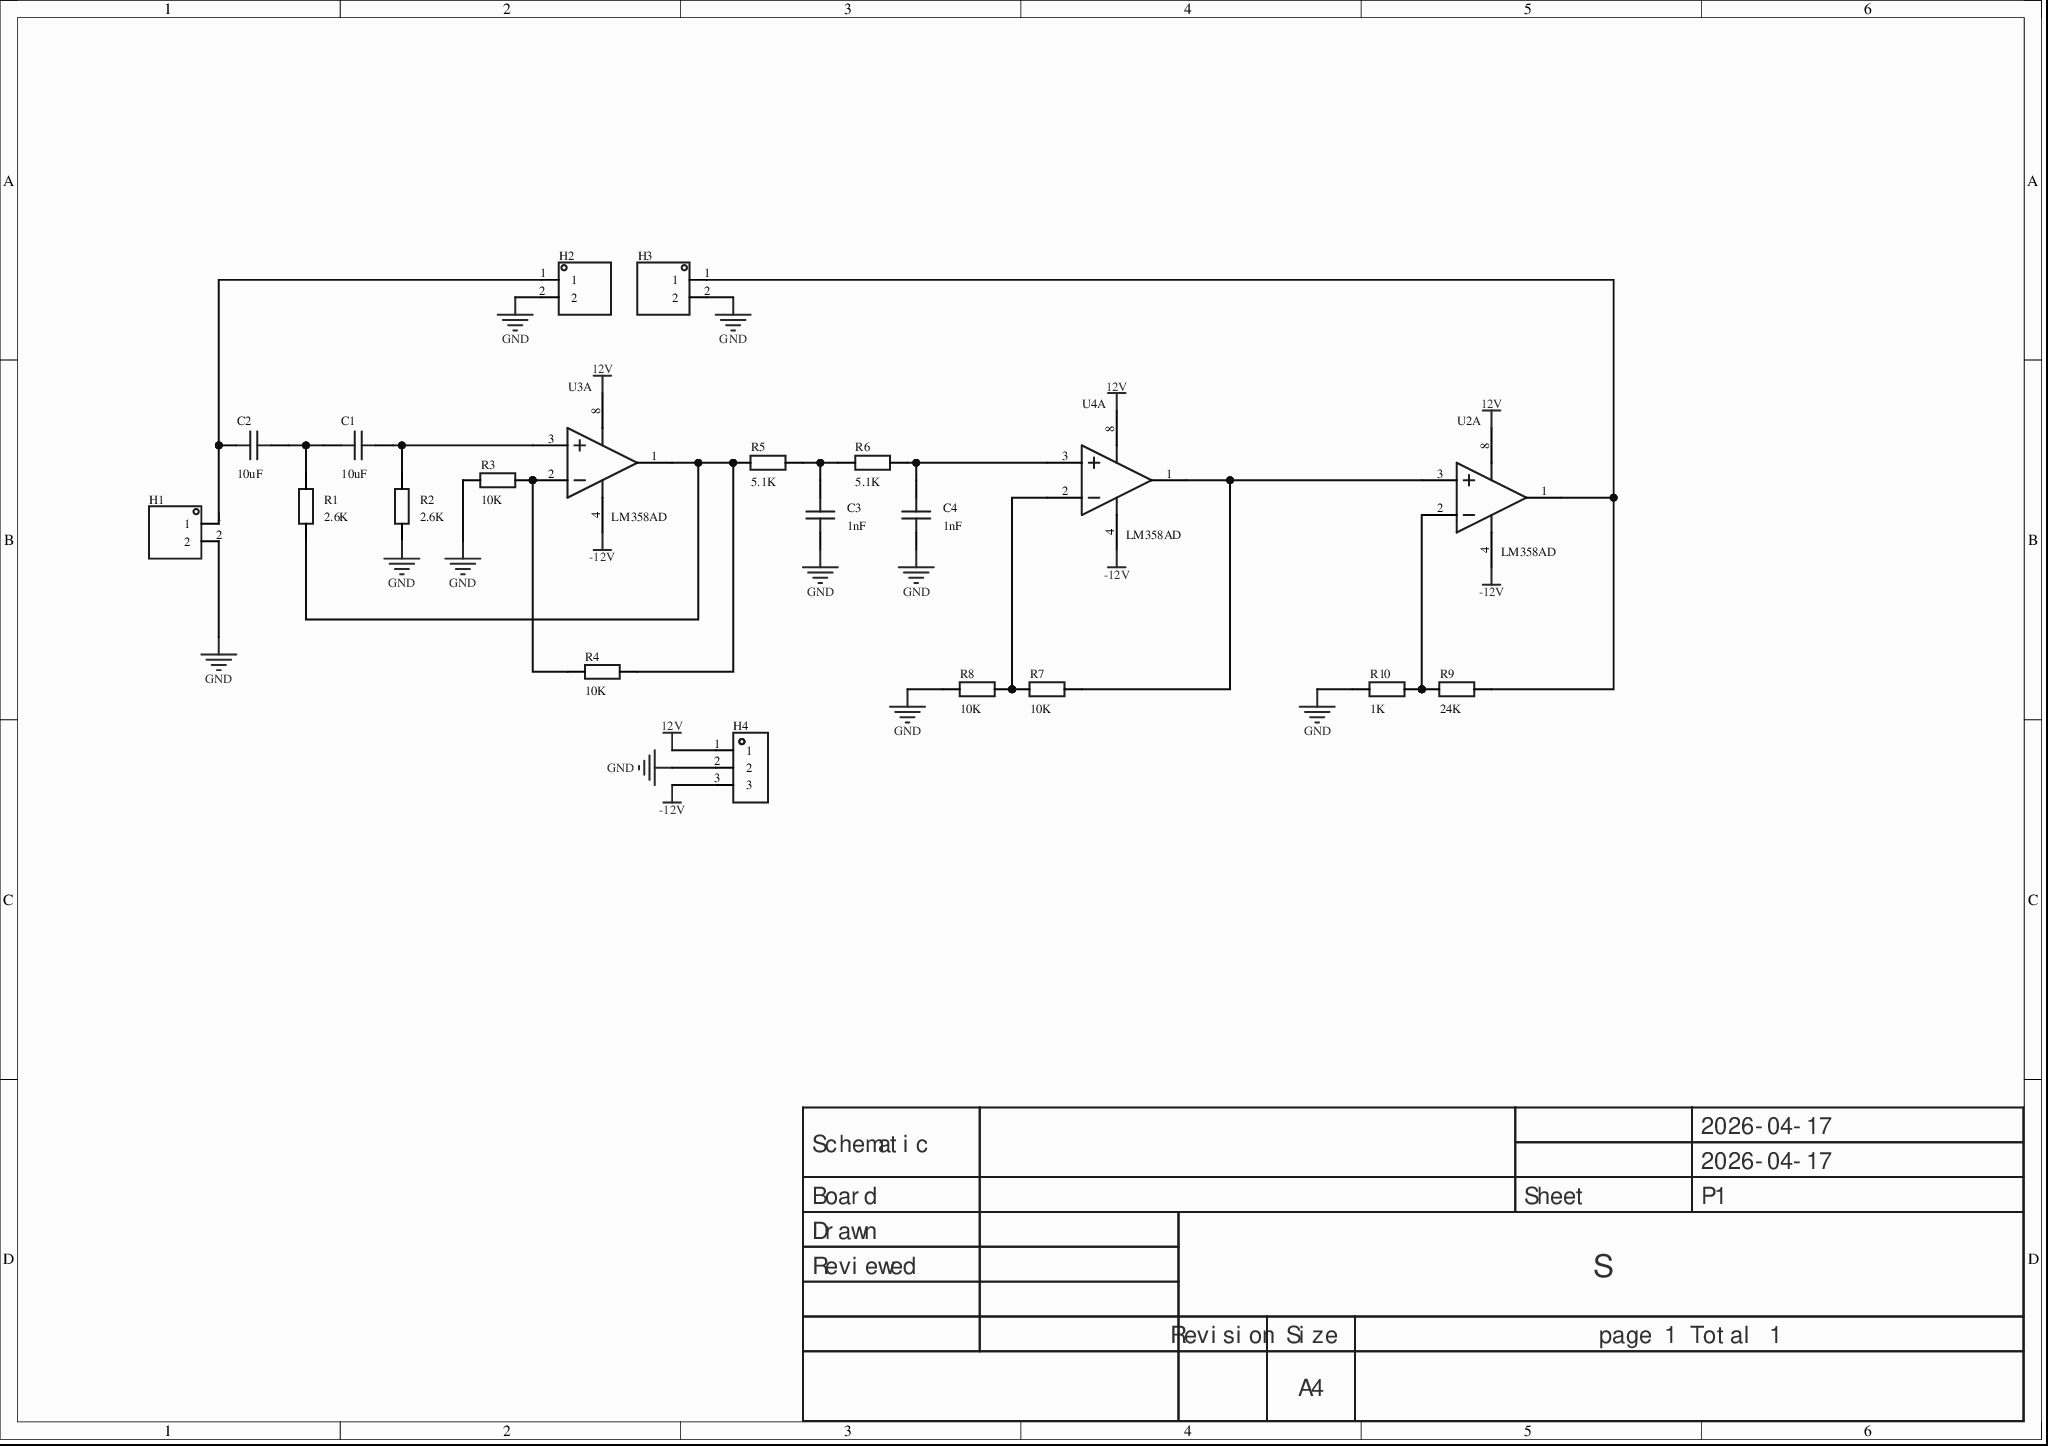
[diagram p0: MISC51939-3.schdoc]
# Altium project MISC51939-2.PrjPcb
1 sheet, 21 parts. Net scope: global (net labels, ports and power ports of the same name join across sheets).
Board file: MISC51939.pcbdoc

## Sheet MISC51939-3.schdoc
size 297 x 209 mm; Version: V1.0; @Project Name: MISC51939; @Update Date: 2026-04-17; @Create Date: 2026-04-17; @Board Name: MISC51939; @Create Time: 21:21:57; @Page Count: 1; @Page No: 1; @Schematic Name: MISC51939; @Update Time: 21:21:57; Size: A4

### Parts
C1  10uF  [C0805]
C2  10uF  [C0805]
C3  1nF  [C0805]
C4  1nF  [C0805]
H1  (no value)  [HDR-TH_2P-P2.54-V-M-1]
H2  (no value)  [HDR-TH_2P-P2.54-V-M-1]
H3  (no value)  [HDR-TH_2P-P2.54-V-M-1]
H4  (no value)  [HDR-TH_3P-P2.54-V-M]
R1  2.6K  [R0805]
R2  2.6K  [R0805]
R3  10K  [R0805]
R4  10K  [R0805]
R5  5.1K  [R0805]
R6  5.1K  [R0805]
R7  10K  [R0805]
R8  10K  [R0805]
R9  24K  [R0805]
R10  1K  [R0805]
U2  LM358AD  [PDIP-8_L9.5-W6.4-P2.54-LS7.6-BL]  (part A of 2)
U3  LM358AD  [PDIP-8_L9.5-W6.4-P2.54-LS7.6-BL]  (part A of 2)
U4  LM358AD  [PDIP-8_L9.5-W6.4-P2.54-LS7.6-BL]  (part A of 2)

### Nets
12V: H4.1 U2.8(V+) U3.8(V+) U4.8(V+)
-12V: H4.3 U2.4(V-) U3.4(V-) U4.4(V-)
GND: C3.1 C4.1 H1.2 H2.2 H3.2 H4.2 R2.1 R3.1 R8.1 R10.1
NetC1_1: C1.1 C2.2 R1.2
NetC1_2: C1.2 R2.2 U3.3(IN1-)
NetC2_1: C2.1 H1.1 H2.1
NetC3_2: C3.2 R5.2 R6.1
NetC4_2: C4.2 R6.2 U4.3(IN1-)
NetH3_1: H3.1 R9.2 U2.1(OUT1)
NetR1_1: R1.1 R4.2 R5.1 U3.1(OUT1)
NetR3_2: R3.2 R4.1 U3.2(IN1+)
NetR7_1: R7.1 R8.2 U4.2(IN1+)
NetR7_2: R7.2 U2.3(IN1-) U4.1(OUT1)
NetR9_1: R9.1 R10.2 U2.2(IN1+)

### Notes on the sheet
- 2026-04-17
- Schematic
- Board
- Sheet
- P1
- Drawn
- Reviewed
- S
- Revision
- Size
- A4
- page 1 Total 1

### Library data of the parts
C1-C4 = CAP_0805: Symbol: Capacitance; ConvertToPcb: yes; ModelId: 1ba041120af144c991958decab20d2410819f05c4eef4c71ace90d822a990e87; ModelName: C0805_L2.0-W1.3-H1.3; ModelTransform: 78.74,51.181,0,0,0,0,0,0.0005,0; Device: CAP_0805; AddInBom: yes; Supplier Footprint: 0805; FootprintName: C0805
  C1 C2: Value: 10uF
  C3 C4: Value: 1nF
H1-H3 = HDR-M_2.54_1x2P: Symbol: 210S-1*2P L=11.6MMGold-plated black; ConvertToPcb: yes; ModelId: 79b2e9f2d70a4d68a1b7098f27c6d4c50819f05c4eef4c71ace90d822a990e87; ModelName: HDR-M-2.54_1x2; ModelTransform: 200,100,0,0,0,0,0,0,-118.11; Device: HDR-M_2.54_1x2P; AddInBom: yes; SupplierPart: C124375; Supplier Footprint: 插件; FootprintName: HDR-TH_2P-P2.54-V-M-1
H4 = HDR-M_2.54_1x3P: AddInBom: yes; ModelId: bb473b6d38ff42a99216a4fcdbdcc4cb0819f05c4eef4c71ace90d822a990e87; ModelName: HDR-TH_3P-P2.54-M-LI-1X3P; ModelTransform: 300.03877,100,0,0,0,0,0,0,-118.11; Symbol: HDR-M_2.54_1x3P; Device: HDR-M_2.54_1x3P; ConvertToPcb: yes; FootprintName: HDR-TH_3P-P2.54-V-M; SupplierPart: C2937625; Supplier Footprint: 插件
R1-R10 = Res_0805: Symbol: Resistor; ConvertToPcb: yes; ModelId: 37a81e68749a4138bd2dfa6897b24b850819f05c4eef4c71ace90d822a990e87; ModelName: R0805_L2.0-W1.3-H0.6; ModelTransform: 78.74,51.181,0,0,0,0,0,-0.0005,0; Device: Res_0805; AddInBom: yes; Supplier Footprint: 0805; FootprintName: R0805
  R1 R2: Value: 2.6K
  R3 R4 R7 R8: Value: 10K
  R5 R6: Value: 5.1K
  R9: Value: 24K
  R10: Value: 1K
U2 U4 = CA3240-DIP-8: Amplifier count: 2; Rail-to-rail: -; Gain bandwidth product (GBW): -; Input offset voltage (Vos): -; Slew rate (SR): -; Input bias current (Ib): -;; Manufacturer: DDF(鼎德丰); Symbol: CA3240-DIP-8_1; Relevance: []; 3D Model: 3e425cb880f24207aa7fdd5a34feb4550819f05c4eef4c71ace90d822a990e87; 3D Model Transform: 372.4402,312.5978,0,0,0,0,0,0,-129.921; Number of Channels: 2; Output Current: 40mA; AddInBom: yes; Device: CA3240-DIP-8; Manufacturer Part: LM358AD; LCSC Part Name: CA3240-DIP-8; Supplier Part: C53199143; Supplier Footprint: DIP-8; JLCPCB Part Class: Extended Part; Datasheet: https://item.szlcsc.com/datasheet/CA3240-DIP-8/56225186.html; Supplier: LCSC; Maximum Power Supply Range (Vdd-Vss): -; Rail to Rail: -; Gain Bandwidth Product: -; Vos - Input Offset Voltage: -; Input Offset Voltage Drift(Vos TC): -; Slew Rate: -; Ib - Input Bias Current: -; Input Offset Current(Ios): -; Input Voltage Noise Density: -; Common Mode Rejection Ratio(CMRR): -; Input offset current drift(Ios TC): -; Quiescent Current: -; Operating Temperature: -20℃~+85℃; Single supply: -; Dual Supply: -; ConvertToPcb: yes; FootprintName: PDIP-8_L9.5-W6.4-P2.54-LS7.6-BL; ModelName: PDIP-8_L9.5-W6.4-P2.54-LS7.6-BL
U3 = CA3240-DIP-8: Amplifier count: 2; Rail-to-rail: -; Gain bandwidth product (GBW): -; Input offset voltage (Vos): -; Slew rate (SR): -; Input bias current (Ib): -;; Manufacturer: DDF(鼎德丰); Symbol: CA3240-DIP-8_1; Relevance: []; AddInBom: yes; ModelId: 3e425cb880f24207aa7fdd5a34feb4550819f05c4eef4c71ace90d822a990e87; ModelTransform: 372.4402,312.5978,0,0,0,0,0,0,-129.921; Number of Channels: 2; Output Current: 40mA; Device: CA3240-DIP-8; Manufacturer Part: LM358AD; LCSC Part Name: CA3240-DIP-8; SupplierPart: C53199143; Supplier Footprint: DIP-8; JLCPCB Part Class: Extended Part; Datasheet: https://item.szlcsc.com/datasheet/CA3240-DIP-8/56225186.html; Supplier: LCSC; ConvertToPcb: yes; FootprintName: PDIP-8_L9.5-W6.4-P2.54-LS7.6-BL; ModelName: PDIP-8_L9.5-W6.4-P2.54-LS7.6-BL; Maximum Power Supply Range (Vdd-Vss): -; Rail to Rail: -; Gain Bandwidth Product: -; Vos - Input Offset Voltage: -; Input Offset Voltage Drift(Vos TC): -; Slew Rate: -; Ib - Input Bias Current: -; Input Offset Current(Ios): -; Input Voltage Noise Density: -; Common Mode Rejection Ratio(CMRR): -; Input offset current drift(Ios TC): -; Quiescent Current: -; Operating Temperature: -20℃~+85℃; Single supply: -; Dual Supply: -